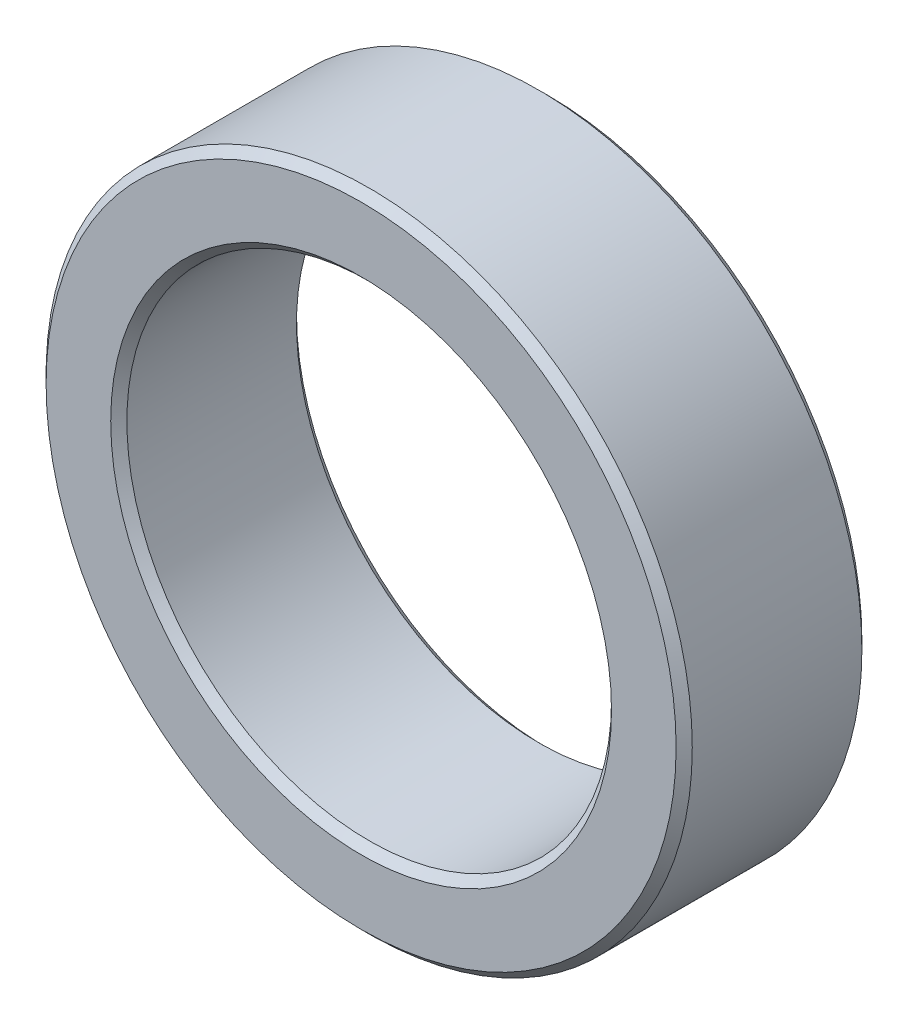
SolidWorks part; units mm, degrees
ref_plane "Front Plane" through (0, 0, 0) normal (0, 0, 1) x (1, 0, 0)
ref_plane "Top Plane" through (0, 0, 0) normal (0, 1, 0) x (1, 0, 0)
ref_plane "Right Plane" through (0, 0, 0) normal (1, 0, 0) x (0, 0, -1)
other "Configuration Table"
sketch "Sketch1" plane through (0, 0, 0) normal (0, 0, 1) x (1, 0, 0)
  circle A0 centre (0, 0) radius 30
  circle A1 centre (0, 0) radius 40
  dimension "D1" = 60
  dimension "D2" = 80
extrude "Boss-Extrude1" add sketch "Sketch1" along normal mid plane 23
chamfer "Chamfer1" distance 1 angle 45 4 edges at (30, 0, -11.5) (40, 0, -11.5) (30, 0, 11.5) (40, 0, 11.5)
